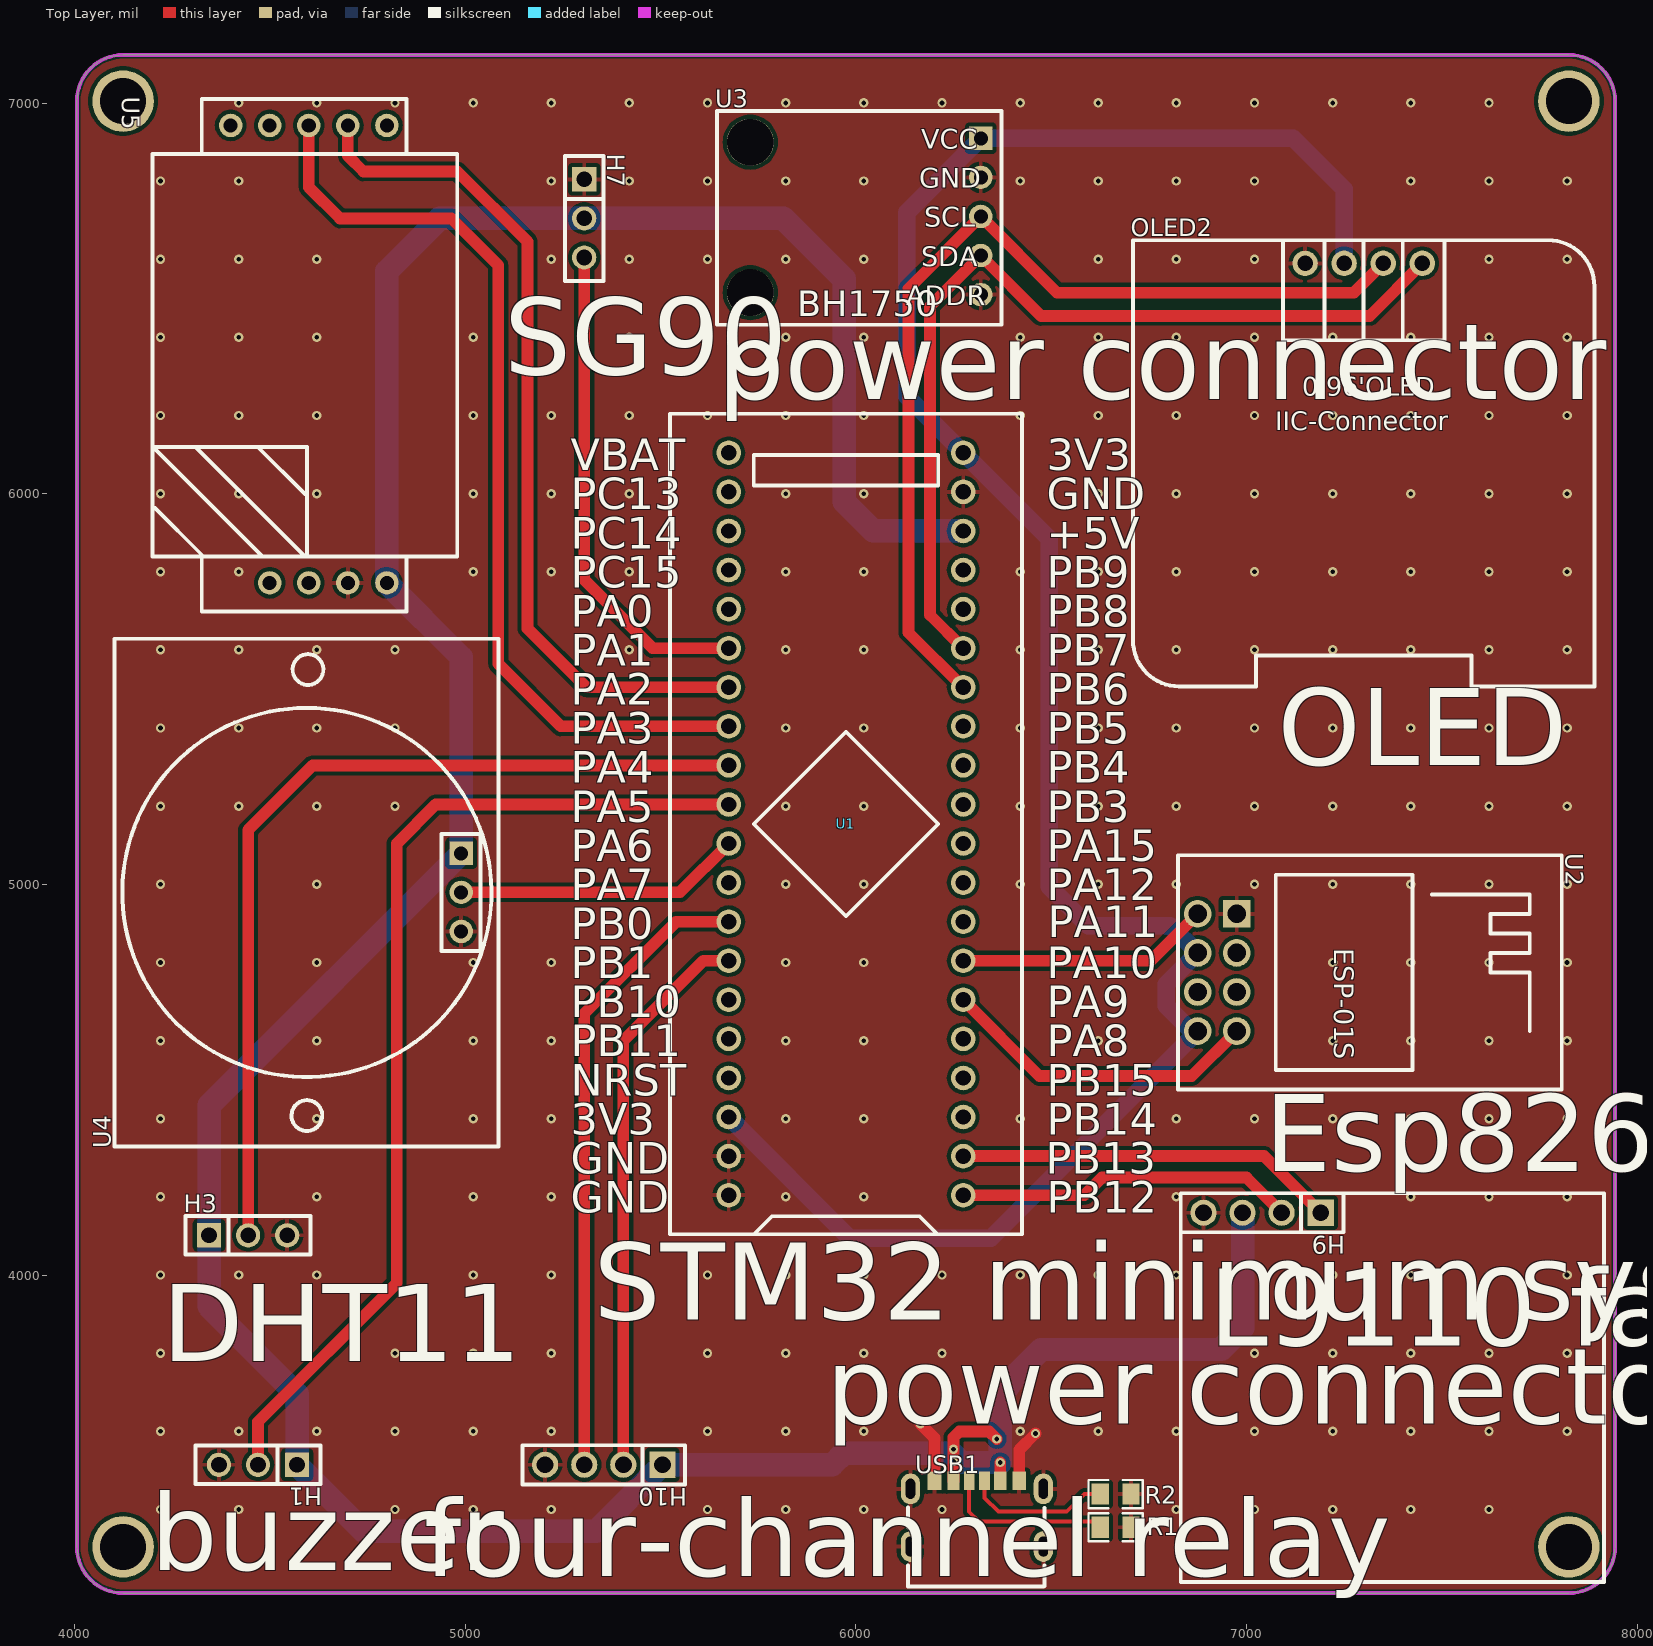
[diagram p0: Top Layer view]
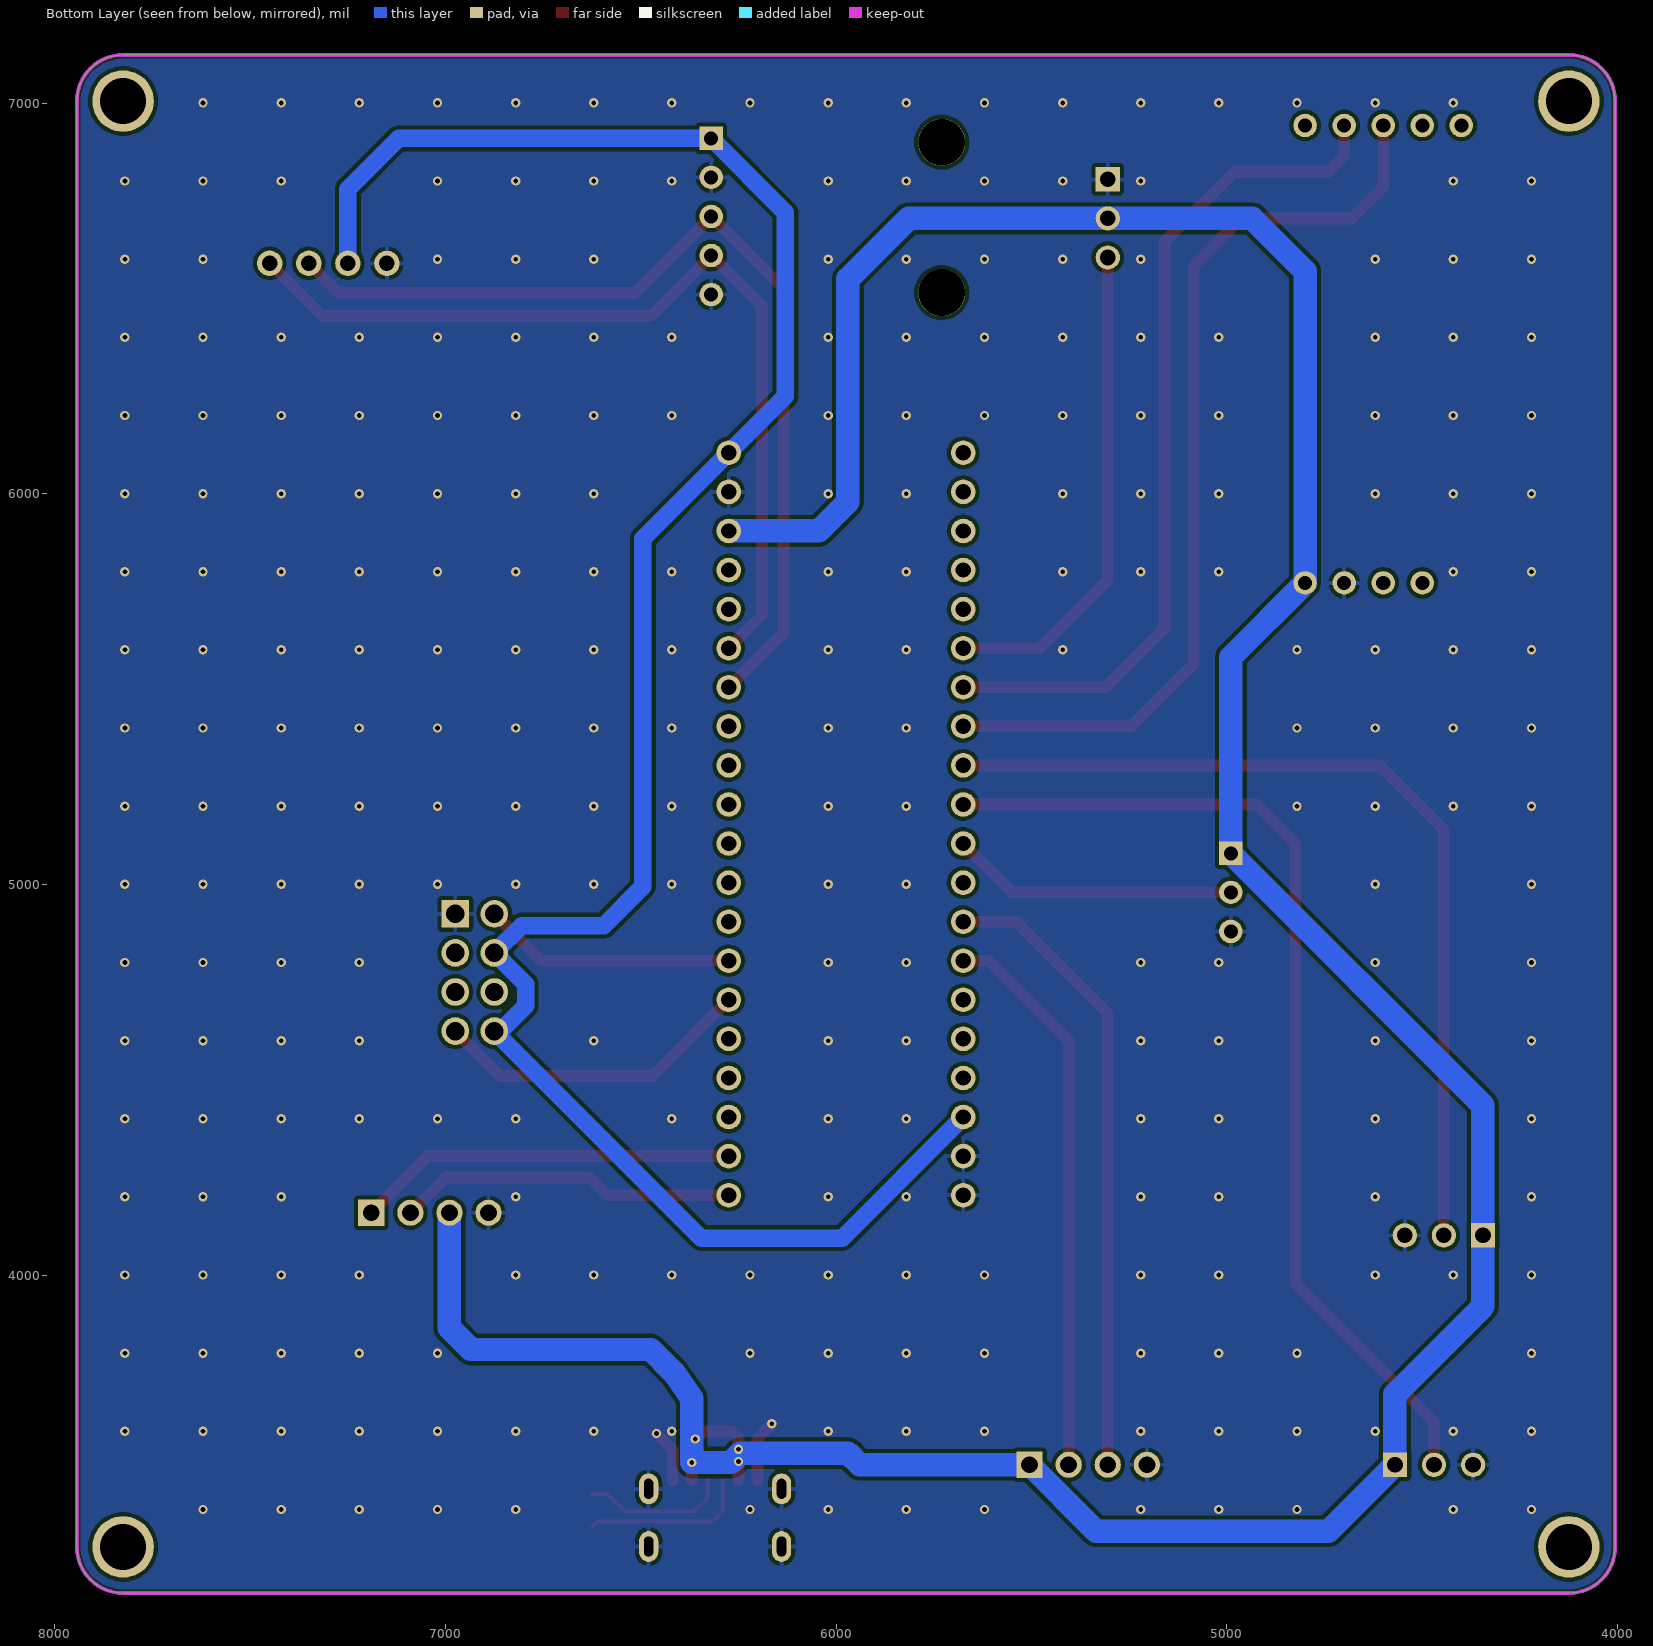
[diagram p1: Bottom Layer view, seen from below]
# Altium PCB MISC89045.pcbdoc
Units mil, origin at the board's own origin, x right, y up, seen from the top; angles counter-clockwise.
Board outline 3937.01 x 3937.01 mil, 2 copper layers (Top Layer, Bottom Layer), stack 62.206 mil thick; 14 components, 39 nets, 106 pads, 273 vias.

## Layer stack, top to bottom
Top Solder Mask Layer: solder mask 0.394, Dk 3.3
Top Layer: signal copper 1.379
Dielectric1: surface 59.449, FR4, Dk 4.5
Bottom Layer: signal copper 1.378
Bottom Solder Mask Layer: solder mask 0.394, Dk 3.3

## Board outline
4124.61,7123.5 ccw(c4124.61,7005.39) 4006.5,7005.39 4006.5,3304.61 ccw(c4124.61,3304.61) 4124.61,3186.5 7825.39,3186.5 ccw(c7825.39,3304.61) 7943.5,3304.61 7943.5,7005.39 ccw(c7825.39,7005.39) 7825.39,7123.5 4124.61,7123.5

## Design rules (kind name [scope] priority, off if disabled: settings)
BoardOutlineClearance copperThickness2oz_1 [All] p2 off: genericclearance=7.99 ignorepadtopadclearanceinfootprint=FALSE except(0: Arc-SplitContinuation Track-SplitContinuation SMDPad-SplitContinuation THPad-SplitContinuation Via-SplitContinuation Fill-SplitContinuation Region-SplitContinuation Poly-SplitContinuation Text-SplitContinuation Hole-SplitContinuation; 5.98: Arc-CutoutEdge Track-CutoutEdge SMDPad-CutoutEdge THPad-CutoutEdge Via-CutoutEdge Text-CutoutEdge; 6.9: Hole-OutlineEdge Hole-CutoutEdge; 10: Poly-OutlineEdge Poly-CutoutEdge; 11.81: Arc-OutlineEdge Track-OutlineEdge SMDPad-OutlineEdge THPad-OutlineEdge Via-OutlineEdge Fill-OutlineEdge Region-OutlineEdge Text-OutlineEdge Fill-CutoutEdge Region-CutoutEdge)
BoardOutlineClearance Plane_innerPlane_1 [All] p4 off: genericclearance=4.02 ignorepadtopadclearanceinfootprint=FALSE except(0: Arc-SplitContinuation Track-SplitContinuation SMDPad-SplitContinuation THPad-SplitContinuation Via-SplitContinuation Fill-SplitContinuation Region-SplitContinuation Poly-SplitContinuation Text-SplitContinuation Hole-SplitContinuation; 5.98: Arc-CutoutEdge Track-CutoutEdge SMDPad-CutoutEdge THPad-CutoutEdge Via-CutoutEdge Text-CutoutEdge; 6.9: Hole-OutlineEdge Hole-CutoutEdge; 10: Poly-OutlineEdge Poly-CutoutEdge; 11.81: Arc-OutlineEdge Track-OutlineEdge SMDPad-OutlineEdge THPad-OutlineEdge Via-OutlineEdge Fill-OutlineEdge Region-OutlineEdge Text-OutlineEdge Fill-CutoutEdge Region-CutoutEdge)
BoardOutlineClearance Copper_copperRegion_1 [All] p6 off: genericclearance=4.02 ignorepadtopadclearanceinfootprint=FALSE except(0: Arc-SplitContinuation Track-SplitContinuation SMDPad-SplitContinuation THPad-SplitContinuation Via-SplitContinuation Fill-SplitContinuation Region-SplitContinuation Poly-SplitContinuation Text-SplitContinuation Hole-SplitContinuation; 5.98: Arc-CutoutEdge Track-CutoutEdge SMDPad-CutoutEdge THPad-CutoutEdge Via-CutoutEdge Text-CutoutEdge; 6.9: Hole-OutlineEdge Hole-CutoutEdge; 10: Poly-OutlineEdge Poly-CutoutEdge; 11.81: Arc-OutlineEdge Track-OutlineEdge SMDPad-OutlineEdge THPad-OutlineEdge Via-OutlineEdge Fill-OutlineEdge Region-OutlineEdge Text-OutlineEdge Fill-CutoutEdge Region-CutoutEdge)
BoardOutlineClearance Copper_copperRegion_copperThickness1oz_1 [All] p8 off: genericclearance=4.02 ignorepadtopadclearanceinfootprint=FALSE except(0: Arc-SplitContinuation Track-SplitContinuation SMDPad-SplitContinuation THPad-SplitContinuation Via-SplitContinuation Fill-SplitContinuation Region-SplitContinuation Poly-SplitContinuation Text-SplitContinuation Hole-SplitContinuation; 5.98: Arc-CutoutEdge Track-CutoutEdge SMDPad-CutoutEdge THPad-CutoutEdge Via-CutoutEdge Text-CutoutEdge; 6.9: Hole-OutlineEdge Hole-CutoutEdge; 10: Poly-OutlineEdge Poly-CutoutEdge; 11.81: Arc-OutlineEdge Track-OutlineEdge SMDPad-OutlineEdge THPad-OutlineEdge Via-OutlineEdge Fill-OutlineEdge Region-OutlineEdge Text-OutlineEdge Fill-CutoutEdge Region-CutoutEdge)
BoardOutlineClearance Copper_copperRegion_Copper_copperRegion_1 [All] p10 off: genericclearance=4.02 ignorepadtopadclearanceinfootprint=FALSE except(0: Arc-SplitContinuation Track-SplitContinuation SMDPad-SplitContinuation THPad-SplitContinuation Via-SplitContinuation Fill-SplitContinuation Region-SplitContinuation Poly-SplitContinuation Text-SplitContinuation Hole-SplitContinuation; 5.98: Arc-CutoutEdge Track-CutoutEdge SMDPad-CutoutEdge THPad-CutoutEdge Via-CutoutEdge Text-CutoutEdge; 6.9: Hole-OutlineEdge Hole-CutoutEdge; 10: Poly-OutlineEdge Poly-CutoutEdge; 11.81: Arc-OutlineEdge Track-OutlineEdge SMDPad-OutlineEdge THPad-OutlineEdge Via-OutlineEdge Fill-OutlineEdge Region-OutlineEdge Text-OutlineEdge Fill-CutoutEdge Region-CutoutEdge)
BoardOutlineClearance copperThickness1oz_1 [All] p12: genericclearance=4.02 ignorepadtopadclearanceinfootprint=FALSE except(0: Arc-SplitContinuation Track-SplitContinuation SMDPad-SplitContinuation THPad-SplitContinuation Via-SplitContinuation Fill-SplitContinuation Region-SplitContinuation Poly-SplitContinuation Text-SplitContinuation Hole-SplitContinuation; 5.98: Arc-CutoutEdge Track-CutoutEdge SMDPad-CutoutEdge THPad-CutoutEdge Via-CutoutEdge Text-CutoutEdge; 6.9: Hole-OutlineEdge Hole-CutoutEdge; 10: Poly-OutlineEdge Poly-CutoutEdge; 11.81: Arc-OutlineEdge Track-OutlineEdge SMDPad-OutlineEdge THPad-OutlineEdge Via-OutlineEdge Fill-OutlineEdge Region-OutlineEdge Text-OutlineEdge Fill-CutoutEdge Region-CutoutEdge)
Clearance copperThickness2oz [All] p1 off: gap=7.99 ignorepadtopadclearanceinfootprint=FALSE except(5.98: SMDPad-Track SMDPad-SMDPad THPad-Track SMDPad-THPad THPad-THPad Track-Via SMDPad-Via THPad-Via Via-Via Fill-SMDPad Region-SMDPad Fill-THPad Region-THPad Fill-Via Region-Via Fill-Fill Fill-Region Region-Region Arc-Track Arc-SMDPad Arc-THPad Arc-Via Fill-Arc Region-Arc Arc-Arc Text-Track SMDPad-Text Text-THPad Text-Via Fill-Text Region-Text Arc-Text Text-Text; 6.9: Hole-Track Hole-SMDPad Hole-THPad Hole-Via Fill-Hole Region-Hole Hole-Arc Hole-Text; 10: Poly-Track Poly-SMDPad Poly-THPad Poly-Via Poly-Fill Poly-Region Poly-Poly Poly-Arc Poly-Text Poly-Hole; 11.81: Fill-Track Region-Track)
Clearance Plane_innerPlane [All] p3 off: gap=4.02 ignorepadtopadclearanceinfootprint=FALSE except(5.98: SMDPad-Track SMDPad-SMDPad THPad-Track SMDPad-THPad THPad-THPad Track-Via SMDPad-Via THPad-Via Via-Via Fill-SMDPad Region-SMDPad Fill-THPad Region-THPad Fill-Via Region-Via Fill-Fill Fill-Region Region-Region Arc-Track Arc-SMDPad Arc-THPad Arc-Via Fill-Arc Region-Arc Arc-Arc Text-Track SMDPad-Text Text-THPad Text-Via Fill-Text Region-Text Arc-Text Text-Text; 6.9: Hole-Track Hole-SMDPad Hole-THPad Hole-Via Fill-Hole Region-Hole Hole-Arc Hole-Text; 10: Poly-Track Poly-SMDPad Poly-THPad Poly-Via Poly-Fill Poly-Region Poly-Poly Poly-Arc Poly-Text Poly-Hole; 11.81: Fill-Track Region-Track)
Clearance Copper_copperRegion [All] p5 off: gap=4.02 ignorepadtopadclearanceinfootprint=FALSE except(5.98: SMDPad-Track SMDPad-SMDPad THPad-Track SMDPad-THPad THPad-THPad Track-Via SMDPad-Via THPad-Via Via-Via Fill-SMDPad Region-SMDPad Fill-THPad Region-THPad Fill-Via Region-Via Fill-Fill Fill-Region Region-Region Arc-Track Arc-SMDPad Arc-THPad Arc-Via Fill-Arc Region-Arc Arc-Arc Text-Track SMDPad-Text Text-THPad Text-Via Fill-Text Region-Text Arc-Text Text-Text; 6.9: Hole-Track Hole-SMDPad Hole-THPad Hole-Via Fill-Hole Region-Hole Hole-Arc Hole-Text; 10: Poly-Track Poly-SMDPad Poly-THPad Poly-Via Poly-Fill Poly-Region Poly-Poly Poly-Arc Poly-Text Poly-Hole; 11.81: Fill-Track Region-Track)
Clearance Copper_copperRegion_copperThickness1oz [All] p7 off: gap=4.02 ignorepadtopadclearanceinfootprint=FALSE except(5.98: SMDPad-Track SMDPad-SMDPad THPad-Track SMDPad-THPad THPad-THPad Track-Via SMDPad-Via THPad-Via Via-Via Fill-SMDPad Region-SMDPad Fill-THPad Region-THPad Fill-Via Region-Via Fill-Fill Fill-Region Region-Region Arc-Track Arc-SMDPad Arc-THPad Arc-Via Fill-Arc Region-Arc Arc-Arc Text-Track SMDPad-Text Text-THPad Text-Via Fill-Text Region-Text Arc-Text Text-Text; 6.9: Hole-Track Hole-SMDPad Hole-THPad Hole-Via Fill-Hole Region-Hole Hole-Arc Hole-Text; 10: Poly-Track Poly-SMDPad Poly-THPad Poly-Via Poly-Fill Poly-Region Poly-Poly Poly-Arc Poly-Text Poly-Hole; 11.81: Fill-Track Region-Track)
Clearance Copper_copperRegion_Copper_copperRegion [All] p9 off: gap=4.02 ignorepadtopadclearanceinfootprint=FALSE except(5.98: SMDPad-Track SMDPad-SMDPad THPad-Track SMDPad-THPad THPad-THPad Track-Via SMDPad-Via THPad-Via Via-Via Fill-SMDPad Region-SMDPad Fill-THPad Region-THPad Fill-Via Region-Via Fill-Fill Fill-Region Region-Region Arc-Track Arc-SMDPad Arc-THPad Arc-Via Fill-Arc Region-Arc Arc-Arc Text-Track SMDPad-Text Text-THPad Text-Via Fill-Text Region-Text Arc-Text Text-Text; 6.9: Hole-Track Hole-SMDPad Hole-THPad Hole-Via Fill-Hole Region-Hole Hole-Arc Hole-Text; 10: Poly-Track Poly-SMDPad Poly-THPad Poly-Via Poly-Fill Poly-Region Poly-Poly Poly-Arc Poly-Text Poly-Hole; 11.81: Fill-Track Region-Track)
Clearance copperThickness1oz [All] p11: gap=4.02 ignorepadtopadclearanceinfootprint=FALSE except(5.98: SMDPad-Track SMDPad-SMDPad THPad-Track SMDPad-THPad THPad-THPad Track-Via SMDPad-Via THPad-Via Via-Via Fill-SMDPad Region-SMDPad Fill-THPad Region-THPad Fill-Via Region-Via Fill-Fill Fill-Region Region-Region Arc-Track Arc-SMDPad Arc-THPad Arc-Via Fill-Arc Region-Arc Arc-Arc Text-Track SMDPad-Text Text-THPad Text-Via Fill-Text Region-Text Arc-Text Text-Text; 6.9: Hole-Track Hole-SMDPad Hole-THPad Hole-Via Fill-Hole Region-Hole Hole-Arc Hole-Text; 10: Poly-Track Poly-SMDPad Poly-THPad Poly-Via Poly-Fill Poly-Region Poly-Poly Poly-Arc Poly-Text Poly-Hole; 11.81: Fill-Track Region-Track)
DiffPairsRouting differentialPair [All] p1: maxlimit=6 minlimit=6 mostfreqgap=6 toplayer_minwidth=5 toplayer_prefwidth=10 toplayer_maxwidth=100 toplayer_mingap=6 toplayer_prefgap=6 toplayer_maxgap=6 bottomlayer_minwidth=5 bottomlayer_prefwidth=10 bottomlayer_maxwidth=100 bottomlayer_mingap=6 bottomlayer_prefgap=6 bottomlayer_maxgap=6 maxuncoupledlength=10
HoleToHoleClearance otherClearance [All] p1: gap=11.81 allowstackedmicrovias=TRUE
Length netLength [All] p1: minlimit=0 maxlimit=0
PasteMaskExpansion pasteMaskExpansion [All] p1: expansion=0
PlaneConnect innerPlane [All] p1: planeconnectstyle=Relief reliefexpansion=20 reliefentries=4 reliefconductorwidth=10 reliefairgap=10
PolygonConnect copperRegion_copperThickness1oz [All] p1 off: connectstyle=Relief reliefconductorwidth=10 reliefentries=4 polygonreliefangle="90 Angle" airgapwidth=10 via.connectstyle=Relief via.reliefconductorwidth=10 via.reliefentries=4 via.polygonreliefangle="90 Angle" via.airgapwidth=10
PolygonConnect copperRegion_Copper_copperRegion [All] p2 off: connectstyle=Relief reliefconductorwidth=10 reliefentries=4 polygonreliefangle="90 Angle" airgapwidth=10 via.connectstyle=Relief via.reliefconductorwidth=10 via.reliefentries=4 via.polygonreliefangle="90 Angle" via.airgapwidth=10
PolygonConnect copperRegion [All] p3: connectstyle=Relief reliefconductorwidth=10 reliefentries=4 polygonreliefangle="90 Angle" airgapwidth=10 via.connectstyle=Relief via.reliefconductorwidth=10 via.reliefentries=4 via.polygonreliefangle="90 Angle" via.airgapwidth=10
RoutingVias viaSize [All] p1: holewidth=12.01 width=24.02 viastyle="Through Hole" minholewidth=11.81 minwidth=19.68 maxholewidth=248.03 maxwidth=393.7
SolderMaskExpansion solderMaskExpansion [IsVia] p1: expansion=-1000 istentingtop=TRUE
SolderMaskExpansion solderMaskExpansion [All] p2: expansion=2 istentingtop=FALSE
Width copperThickness2oz_2 [All] p1 off: maxlimit=100 minlimit=8 preferedwidth=10
Width copperThickness1oz_2 [All] p2: maxlimit=100 minlimit=5 preferedwidth=10

## Components (designator, comment, footprint, x,y, rotation, side; value= is the part's Value field where it differs from the comment)
H1 "" HDR-TH_3P-P2.54-V-F 4470,3515 r180 top
H3 "" HDR-TH_3P-P2.54-V-F 4444.74,4102.31 r0 top
H7 "" HDR-TH_3P-P2.54-V-F 5305,6705 r270 top
H9 "" HDR-TH_4P-P2.54-V-F 7040,4160 r180 top
H10 "" HDR-TH_4P-P2.54-V-F 5355,3515 r180 top
OLED2 "" 0.96OLED_4P 7300,6590 r0 top
R1 "5.1K" R0805 6665,3355 r0 top
R2 "5.1K" R0805 6665,3440 r0 top
U1 "STM32F103C8T6-Card" CONN-TH_L53.3-W22.9_STM32F103C8T6-CARD 5975,5155 r90 top
U2 "ESP-01S" WIFIM-TH_ESP-01S 6925,4775 r270 top
U3 "" BH1750光照传感器 6060,6700 r0 top
U4 "" HC-SR501_W32_H24 4990,4980 r90 top
U5 "" MH-Z19C-9PIN 4850,5840 r270 top
USB1 "" "USB_ TYPE-C-6P" 6305,3390 r0 top

## Footprints (in the part's own frame and the unit in brackets; to place one, negate y for a bottom-side part, rotate by r counter-clockwise, add the part's x,y. Pads: shape width x height; smd on the part's side, far side on the other; paste and mask are expansions set on the pad)
0.96OLED_4P [mm]
  round 1.65 hole 1 copper offset 0,0: 1(-3.81,-0.001) 2(-1.27,0.002) 3(1.27,0.002) 4(3.81,0.002)
  silkscreen extent -15,-27.5 15,1.5
BH1750光照传感器 [mil]
  rect 60x60 hole 36: 1(260,210)
  round 60 hole 36: 2(260,110) 3(260,10) 4(260,-90) 5(260,-190)
  round 120 hole 120 unplated: ""(-330,-185) ""(-330,200)
  silkscreen extent -415,-267 313,280
CONN-TH_L53.3-W22.9_STM32F103C8T6-CARD [mm]
  round 1.6 hole 1: 1(-24.13,-7.62) 2(-21.59,-7.62) 3(-19.05,-7.62) 4(-16.51,-7.62) 5(-13.97,-7.62) 6(-11.43,-7.62) 7(-8.89,-7.62) 8(-6.35,-7.62) 9(-3.81,-7.62) 10(-1.27,-7.62) 11(1.27,-7.62) 12(3.81,-7.62) 13(6.35,-7.62) 14(8.89,-7.62) 15(11.43,-7.62) 16(13.97,-7.62) 17(16.51,-7.62) 18(19.05,-7.62) 19(21.59,-7.62) 20(24.13,-7.62) 21(24.13,7.62) 22(21.59,7.62) 23(19.05,7.62) 24(16.51,7.62) 25(13.97,7.62) 26(11.43,7.62) 27(8.89,7.62) 28(6.35,7.62) 29(3.81,7.62) 30(1.27,7.62) 31(-1.27,7.62) 32(-3.81,7.62) 33(-6.35,7.62) 34(-8.89,7.62) 35(-11.43,7.62) 36(-13.97,7.62) 37(-16.51,7.62) 38(-19.05,7.62) 39(-21.59,7.62) 40(-24.13,7.62)
  silkscreen extent -26.67,-11.43 26.67,11.43
HC-SR501_W32_H24 [mil]
  rect 60x60 hole 36: 1(100,0)
  round 60 hole 36: 2(0,0) 3(-100,0)
  silkscreen extent -650,-95 649,887
HDR-TH_3P-P2.54-V-F [mil]
  rect 62x62 hole 40.16: 1(-100,0)
  round 62 hole 40.16: 2(0,0) 3(100,0)
  silkscreen extent -160,-49 160,49
HDR-TH_4P-P2.54-V-F [mm]
  rect 1.7x1.7 hole 1.1: 1(-3.81,0)
  round 1.7 hole 1.1: 2(-1.27,0) 3(1.27,0) 4(3.81,0)
  silkscreen extent -5.29,-1.27 5.29,1.27
MH-Z19C-9PIN [mil]
  round 60 hole 36: 1(67.91,-50) 2(67.91,-150) 3(67.91,-250) 4(67.91,-350) 5(-1102.91,-450) 6(-1102.91,-350) 7(-1102.91,-250) 8(-1102.91,-150) 9(-1102.91,-50)
  silkscreen extent -1171,-650 141,130
R0805 [mm]
  rect 1.133x1.377 smd paste-100 mask+0.051: 1(-1,0) 2(1,0)
  silkscreen extent -1.76,-0.92 1.76,0.92
"USB_ TYPE-C-6P" [mm]
  oval 1.25x2 hole 0.6 slot 1.3 at 90 deg paste+0 mask+0.05: 7(-4.193,1.611) 8(4.447,1.611) 9(-4.193,-2.139) 10(4.447,-2.139)
  rect 0.7x1.2 smd paste-100 mask+0.05: A5(-0.373,2.139) B5(0.627,2.139)
  rect 0.8x1.2 smd paste-100 mask+0.05: A9(1.647,2.139) B9(-1.393,2.139)
  rect 0.9x1.2 smd paste-100 mask+0.05: A12(2.877,2.139) B12(-2.623,2.139)
  silkscreen extent -4.34,-4.75 4.52,0.39
WIFIM-TH_ESP-01S [mm]
  rect 1.8x1.8 hole 1.2: 1(-3.81,1.27)
  round 1.8 hole 1.2: 2(-1.27,1.27) 3(1.27,1.27) 4(3.81,1.27) 5(3.81,-1.27) 6(1.27,-1.27) 7(-1.27,-1.27) 8(-3.81,-1.27)
  silkscreen extent -7.62,-2.54 7.62,22.4

## Free pads (board coordinates)
  round 157.48 hole 118.11: 1(4124.61,7005.39) 1(4124.61,3304.61) 1(7825.39,7005.39) 1(7825.39,3304.61)

## Via types
v1: diameter 24.02, hole 12, Top Layer to Bottom Layer, 273 vias

## Nets (pads, with @x,y where several pads share a name; then routed paths per layer and width w, separated by ;. In a path a pad name is that pad's centre, name@x,y a point inside that pad or via, vN(x,y) a via of type N, cw(c..) or ccw(c..) an arc to the next point about the centre after c; other vN are vias at no path point)
$1N17266: R1.1 USB1.A5 | length 431.3
  Top Layer w10: USB1.A5 6290.32,3394.68 6315,3370 6610.63,3370 R1.1
$1N17267: R2.1 USB1.B5 | length 373.1
  Top Layer w10: USB1.B5 6329.69,3430.31 6365,3395 6540,3395 6585,3440 R2.1
+5V: H1.1 H3.1 H7.2 H9.3 H10.1 U1.18 U4.1 U5.1 USB1.A9 USB1.B9 | length 9096.7
  Top Layer w30: USB1.B9 v1(6250.16,3523.33) v1(6250.16,3554.41) 6250.16,3585.16 6265,3600 6341.57,3600 v1(6360.67,3580.9) ; USB1.A9 v1(6369.84,3520.8)
  Bottom Layer w60: U1.18 6045,5905 5970,5980 5970,6550 5815,6705 H7.2 4935,6705 4800,6570 U5.1 4990,5582.08 U4.1 4344.74,4434.74 H3.1 4344.74,3920.26 4570,3695 H1.1 4740,3345 5335,3345 H10.1 5940,3515 5970,3545 6245,3545 6269.2,3520.8 v1(6369.84,3520.8) 6369.84,3684.84 6415,3750 6475,3810 6935,3810 6990,3865 H9.3
GND: H1.3 H3.3 H7.1 H9.4 H10.4 OLED2.1 R1.2 R2.2 U1.19 U1.39 U1.40 U2.1 U3.2 U3.5 U4.3 U5.2 USB1.7 USB1.8 USB1.9 USB1.10 USB1.A12 USB1.B12 | length 299.1
  Top Layer w30: v1(6165,3620) 6201.73,3583.27 USB1.B12 ; USB1.A12 6418.27,3553.27 v1(6460,3595)
  other v1: 4220.6,3400.6 4420.6,3400.6 4820.6,3400.6 5020.6,3400.6 5220.6,3400.6 5620.6,3400.6 5820.6,3400.6 6020.6,3400.6 6220.6,3400.6 6820.6,3400.6 7020.6,3400.6 7220.6,3400.6 7420.6,3400.6 7620.6,3400.6 4220.6,3600.6 4420.6,3600.6 4620.6,3600.6 4820.6,3600.6 5020.6,3600.6 5220.6,3600.6 5620.6,3600.6 5820.6,3600.6 6020.6,3600.6 6420.6,3600.6 6620.6,3600.6 6820.6,3600.6 7020.6,3600.6 7220.6,3600.6 7420.6,3600.6 7620.6,3600.6 7820.6,3600.6 4220.6,3800.6 4820.6,3800.6 5020.6,3800.6 5220.6,3800.6 5620.6,3800.6 5820.6,3800.6 6020.6,3800.6 6220.6,3800.6 7020.6,3800.6 7220.6,3800.6 7420.6,3800.6 7620.6,3800.6 7820.6,3800.6 4220.6,4000.6 4420.6,4000.6 4620.6,4000.6 5020.6,4000.6 5220.6,4000.6 5620.6,4000.6 5820.6,4000.6 6020.6,4000.6 6220.6,4000.6 6420.6,4000.6 6620.6,4000.6 6820.6,4000.6 7220.6,4000.6 7420.6,4000.6 7620.6,4000.6 7820.6,4000.6 4220.6,4200.6 4620.6,4200.6 5020.6,4200.6 5220.6,4200.6 5820.6,4200.6 6020.6,4200.6 6820.6,4200.6 7420.6,4200.6 7620.6,4200.6 7820.6,4200.6 4220.6,4400.6 4620.6,4400.6 5020.6,4400.6 5220.6,4400.6 5820.6,4400.6 6020.6,4400.6 6420.6,4400.6 6820.6,4400.6 7020.6,4400.6 7220.6,4400.6 7420.6,4400.6 7620.6,4400.6 7820.6,4400.6 4220.6,4600.6 4620.6,4600.6 5020.6,4600.6 5220.6,4600.6 5820.6,4600.6 6020.6,4600.6 6620.6,4600.6 7220.6,4600.6 7420.6,4600.6 7620.6,4600.6 7820.6,4600.6 4220.6,4800.6 4620.6,4800.6 5020.6,4800.6 5220.6,4800.6 5820.6,4800.6 6020.6,4800.6 7220.6,4800.6 7420.6,4800.6 7620.6,4800.6 7820.6,4800.6 4220.6,5000.6 4620.6,5000.6 5820.6,5000.6 6020.6,5000.6 6420.6,5000.6 6620.6,5000.6 6820.6,5000.6 7020.6,5000.6 7220.6,5000.6 7420.6,5000.6 7620.6,5000.6 7820.6,5000.6 4220.6,5200.6 4420.6,5200.6 4620.6,5200.6 4820.6,5200.6 5820.6,5200.6 6020.6,5200.6 6420.6,5200.6 6620.6,5200.6 6820.6,5200.6 7020.6,5200.6 7220.6,5200.6 7420.6,5200.6 7620.6,5200.6 7820.6,5200.6 4220.6,5400.6 4420.6,5400.6 4620.6,5400.6 4820.6,5400.6 5820.6,5400.6 6020.6,5400.6 6420.6,5400.6 6620.6,5400.6 6820.6,5400.6 7020.6,5400.6 7220.6,5400.6 7420.6,5400.6 7620.6,5400.6 7820.6,5400.6 4220.6,5600.6 4420.6,5600.6 4620.6,5600.6 4820.6,5600.6 5420.6,5600.6 5820.6,5600.6 6020.6,5600.6 6420.6,5600.6 6620.6,5600.6 6820.6,5600.6 7020.6,5600.6 7220.6,5600.6 7420.6,5600.6 7620.6,5600.6 7820.6,5600.6 4220.6,5800.6 4420.6,5800.6 5020.6,5800.6 5220.6,5800.6 5420.6,5800.6 5820.6,5800.6 6020.6,5800.6 6420.6,5800.6 6620.6,5800.6 6820.6,5800.6 7020.6,5800.6 7220.6,5800.6 7420.6,5800.6 7620.6,5800.6 7820.6,5800.6 4220.6,6000.6 4420.6,6000.6 4620.6,6000.6 5020.6,6000.6 5220.6,6000.6 5420.6,6000.6 5820.6,6000.6 6020.6,6000.6 6620.6,6000.6 6820.6,6000.6 7020.6,6000.6 7220.6,6000.6 7420.6,6000.6 7620.6,6000.6 7820.6,6000.6 4220.6,6200.6 4420.6,6200.6 4620.6,6200.6 5020.6,6200.6 5220.6,6200.6 5420.6,6200.6 5620.6,6200.6 5820.6,6200.6 6020.6,6200.6 6420.6,6200.6 6620.6,6200.6 6820.6,6200.6 7020.6,6200.6 7220.6,6200.6 7420.6,6200.6 7620.6,6200.6 7820.6,6200.6 4220.6,6400.6 4420.6,6400.6 4620.6,6400.6 5020.6,6400.6 5220.6,6400.6 5420.6,6400.6 5620.6,6400.6 5820.6,6400.6 6020.6,6400.6 6420.6,6400.6 6620.6,6400.6 6820.6,6400.6 7020.6,6400.6 7220.6,6400.6 7420.6,6400.6 7620.6,6400.6 7820.6,6400.6 4220.6,6600.6 4420.6,6600.6 4620.6,6600.6 5220.6,6600.6 5420.6,6600.6 5620.6,6600.6 5820.6,6600.6 6020.6,6600.6 6620.6,6600.6 6820.6,6600.6 7020.6,6600.6 7620.6,6600.6 7820.6,6600.6 4220.6,6800.6 4420.6,6800.6 5220.6,6800.6 5420.6,6800.6 5620.6,6800.6 5820.6,6800.6 6020.6,6800.6 6420.6,6800.6 6620.6,6800.6 6820.6,6800.6 7020.6,6800.6 7420.6,6800.6 7620.6,6800.6 7820.6,6800.6 4420.6,7000.6 4620.6,7000.6 4820.6,7000.6 5020.6,7000.6 5220.6,7000.6 5420.6,7000.6 5620.6,7000.6 5820.6,7000.6 6020.6,7000.6 6220.6,7000.6 6420.6,7000.6 6620.6,7000.6 6820.6,7000.6 7020.6,7000.6 7220.6,7000.6 7420.6,7000.6 7620.6,7000.6
NRST: U1.37
PA0: U1.25
PA1: H7.3 U1.26 | length 1267.5
  Top Layer w30: H7.3 5305,5780 5480,5605 U1.26
PA2: U1.27 U5.8 | length 2196.2
  Top Layer w30: U5.8 4700,6865 4740,6825 4980,6825 5160,6645 5160,5655 5310,5505 U1.27
PA3: U1.28 U5.7 | length 2402
  Top Layer w30: U5.7 4600,6785 4680,6705 4965,6705 5085,6585 5085,5565 5245,5405 U1.28
PA4: H3.2 U1.29 | length 2336.1
  Top Layer w30: H3.2 4444.74,5139.74 4610,5305 U1.29
PA5: H1.2 U1.30 | length 2628.5
  Top Layer w30: H1.2 4470,3625 4825,3980 4825,5105 4925,5205 U1.30
PA6: U1.31 U4.2 | length 736.8
  Top Layer w30: U4.2 5550,4980 U1.31
PA7: U1.32
PA8: U1.5
PA9: U1.6 U2.4 | length 828.4
  Top Layer w30: U1.6 6470,4510 6860,4510 U2.4
PA10: U1.7 U2.8 | length 649.7
  Top Layer w30: U1.7 6755,4805 U2.8
PA11: U1.8
PA12: U1.9
PA15: U1.10
PB0: H10.3 U1.33 | length 1622.3
  Top Layer w30: H10.3 5305,4670 5540,4905 U1.33
PB1: H10.2 U1.34 | length 1439.9
  Top Layer w30: H10.2 5405,4600 5610,4805 U1.34
PB3: U1.11
PB4: U1.12
PB5: U1.13
PB6: OLED2.3 U1.14 U3.3 | length 2481.5
  Top Layer w30: U1.14 6135,5645 6135,6525 U3.3 6515,6515 7274.95,6515 OLED2.3@7350,6590.05
PB7: OLED2.4 U1.15 U3.4 | length 2344.2
  Top Layer w30: U1.15 6190,5690 6190,6480 U3.4 6475,6455 7314.95,6455 OLED2.4@7450,6590.05
PB8: U1.16
PB9: U1.17
PB10: U1.35
PB11: U1.36
PB12: H9.2 U1.1 | length 870.9
  Top Layer w30: U1.1 6585,4205 6630,4250 7000,4250 H9.2
PB13: H9.1 U1.2 | length 975.1
  Top Layer w30: U1.2 7045,4305 H9.1
PB14: U1.3
PB15: U1.4
PC13: U1.22
PC14: U1.23
PC15: U1.24
VBAT: U1.21
VCC: OLED2.2 U1.20 U1.38 U2.5 U2.7 U3.1 | length 5592.1
  Bottom Layer w45: U1.38 5985,4095 6345,4095 U2.5 6860,4625 6795,4690 6795,4745 U2.7 6805,4895 6595,4895 6495,4995 6495,5885 U1.20 6130,6250 6130,6720 U3.1 7120,6910 7250,6780 OLED2.2@7250,6590.05
pads on no net: U2.2 U2.3 U2.6 U3. U5.3 U5.4 U5.5 U5.6 U5.9

## Polygon pours and split planes (outlines as drawn)
GND on Bottom Layer (solid, remove dead copper, pour order 2): 3935,7245 3935,3080 8110,3080 8110,7245
GND on Top Layer (solid, remove dead copper, pour order 2): 3410,7415 3410,3000 8340,3000 8340,7415

## Keep-outs
Board Outline Layer:
  the board outline again, w10

## Silkscreen, mask and mechanical layers (free items; w line width, h text height)
Top Silkscreen Layer:
  lines w10: 6831.73,3215 6831.73,4210 7915,4210 7915,3215 6831.73,3215
  text "SG90" at 5100,6305 h196.85
  text "power connector" at 5646.3,6241.57 h196.85
  text "VBAT" at 5270.95,6060 h80
  text "3V3" at 6489.16,6060 h80
  text "PC13" at 5270.95,5960 h80
  text "GND" at 6489.16,5960 h80
  text "PC14" at 5270.95,5860 h80
  text "+5V" at 6489.16,5860 h80
  text "PC15" at 5270.95,5760 h80
  text "PB9" at 6489.16,5760 h80
  text "PA0" at 5270.95,5660 h80
  text "PB8" at 6489.16,5660 h80
  text "PA1" at 5270.95,5560 h80
  text "PB7" at 6489.16,5560 h80
  text "PA2" at 5270.95,5460 h80
  text "PB6" at 6489.16,5460 h80
  text "PA3" at 5270.95,5360 h80
  text "PB5" at 6489.16,5360 h80
  text "OLED" at 7080,5305 h196.85
  text "PA4" at 5270.95,5260 h80
  text "PB4" at 6489.16,5260 h80
  text "PA5" at 5270.95,5160 h80
  text "PB3" at 6489.16,5160 h80
  text "PA6" at 5270.95,5060 h80
  text "PA15" at 6489.16,5060 h80
  text "PA7" at 5270.95,4960 h80
  text "PA12" at 6489.16,4960 h80
  text "PA11" at 6490.95,4865 h80
  text "PB0" at 5270.95,4860 h80
  text "PB1" at 5270.95,4760 h80
  text "PA10" at 6489.16,4760 h80
  text "PB10" at 5270.95,4660 h80
  text "PA9" at 6489.16,4660 h80
  text "PB11" at 5270.95,4560 h80
  text "PA8" at 6489.16,4560 h80
  text "NRST" at 5270.95,4460 h80
  text "PB15" at 6489.16,4460 h80
  text "3V3" at 5270.95,4360 h80
  text "PB14" at 6489.16,4360 h80
  text "Esp8266-01s" at 7046.3,4266.57 h196.85
  text "GND" at 5270.95,4260 h80
  text "PB13" at 6485.95,4260 h80
  text "GND" at 5270.95,4160 h80
  text "PB12" at 6489.16,4160 h80
  text "STM32 minimum system" at 5329.45,3886.57 h196.85
  text "L9110 fan" at 6905,3820 h196.85
  text "DHT11" at 4225,3780 h196.85
  text "power connector" at 5925,3620 h196.85
  text "buzzer" at 4195,3245 h196.85
  text "four-channel relay" at 4895,3230 h196.85